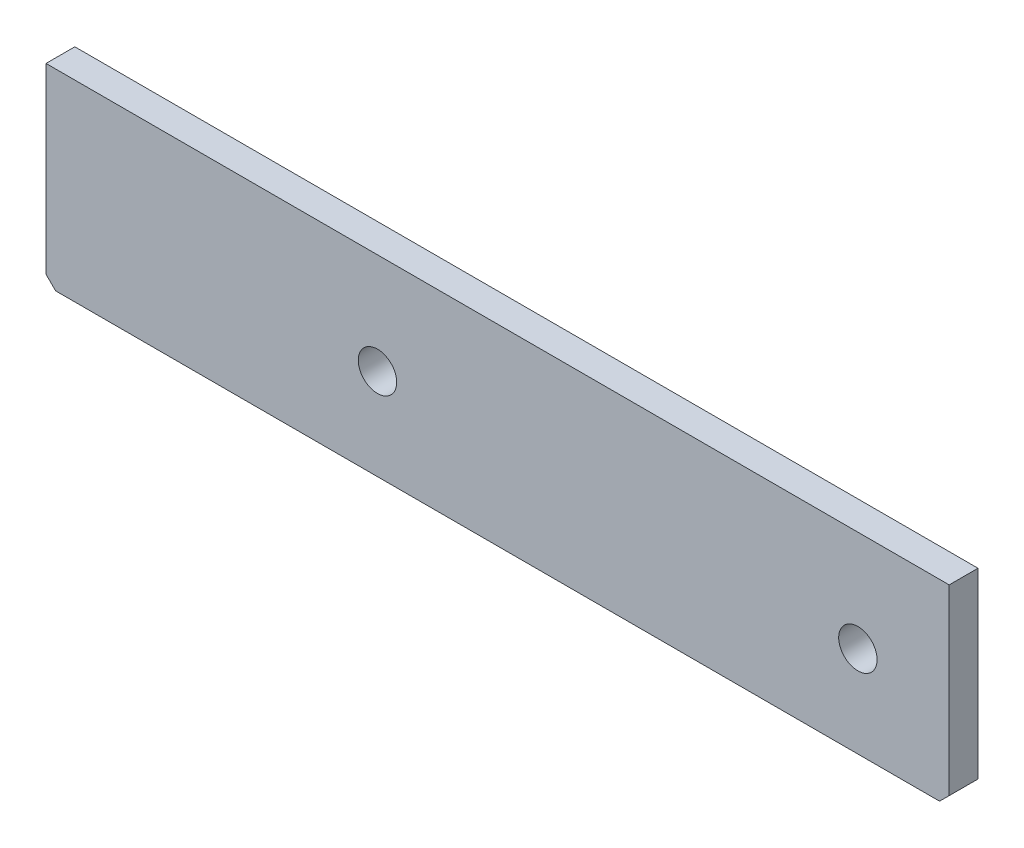
SolidWorks part; units mm, degrees
material "1023 Carbon Steel Plate (SS)"
ref_plane "Front Plane" through (0, 0, 0) normal (0, 0, 1) x (1, 0, 0)
ref_plane "Top Plane" through (0, 0, 0) normal (0, 1, 0) x (1, 0, 0)
ref_plane "Right Plane" through (0, 0, 0) normal (1, 0, 0) x (0, 0, -1)
sketch "Sketch1" plane through (0, 0, 0) normal (0, 0, 1) x (1, 0, 0)
  line L1 (94, 20) -> (-94, 20)
  line L2 (94, 20) -> (94, -20)
  line L3 (94, -20) -> (-94, -20)
  line L4 (-94, 20) -> (-94, -20)
  line L5 (94, 20) -> (-94, -20) construction
  line L6 (94, -20) -> (-94, 20) construction
  point P0 (0, 0)
  dimension "D1" = 188
  dimension "D2" = 40
extrude "Boss-Extrude1" add sketch "Sketch1" along normal blind 6
sketch "Sketch2" plane through (0, 0, 6) normal (0, 0, 1) x (1, 0, 0)
  line L0 (-94, -20) -> (94, -20) construction
  line L1 (-94, 20) -> (-94, -20) construction
  circle A0 centre (-25, -1) radius 4
  circle A1 centre (75, -1) radius 4
  dimension "D1" = 8
  dimension "D2" = 19
  dimension "D3" = 8
  dimension "D4" = 100
  dimension "D5" = 69
extrude "Cut-Extrude1" cut sketch "Sketch2" against normal blind 6
chamfer "Chamfer1" distance 2 angle 45 2 edges at (94, -20, 3) (-94, -20, 3)
